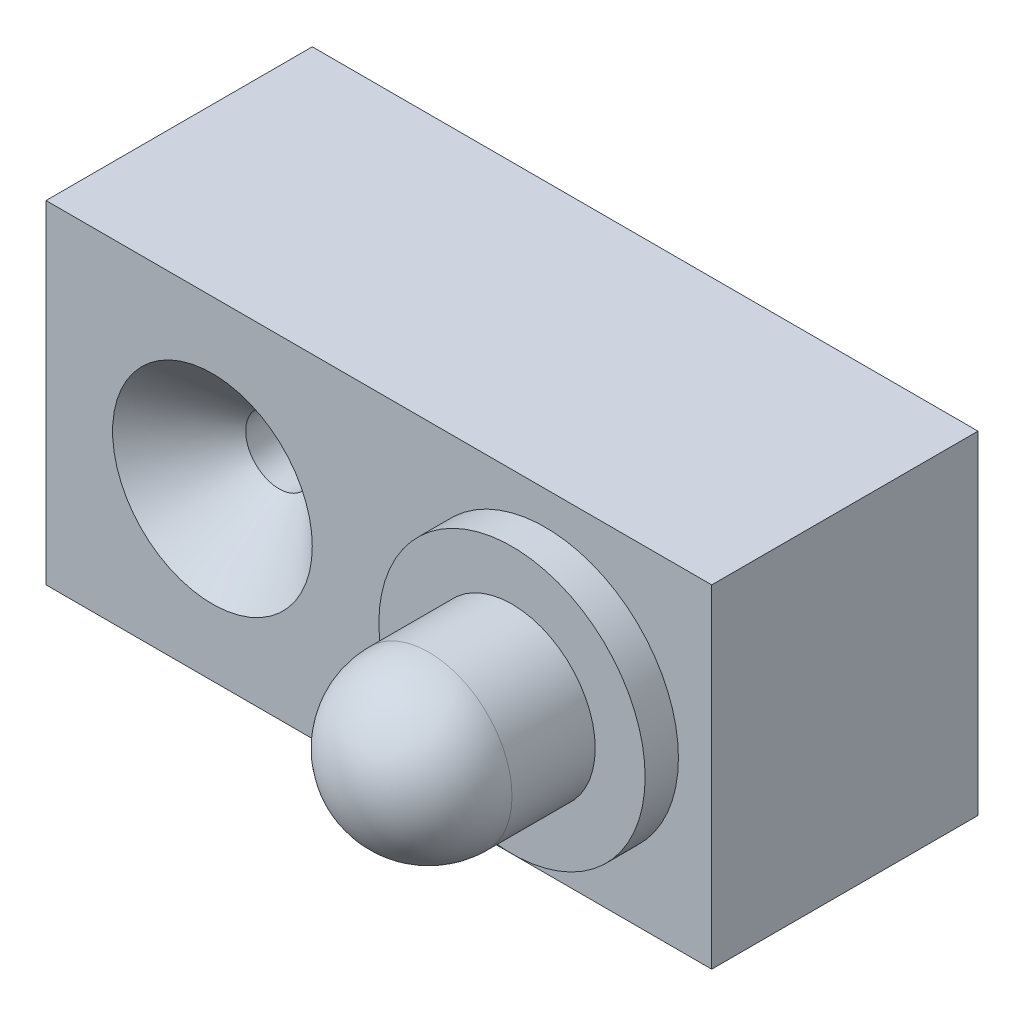
from build123d import *

# Parameters (mm, degrees)
SKETCH_1_W          = 20
SKETCH_1_H          = 10
EXTRUDE_1_DEPTH     = 8
SKETCH_2_R          = 1
CUT_EXTRUDE_1_DEPTH = 8
CHAMFER_1_SIZE      = 2
SKETCH_3_R          = 4
EXTRUDE_2_DEPTH     = 1
SKETCH_4_R          = 2.5
EXTRUDE_3_DEPTH     = 5
FILLET_1_R          = 2.5


with BuildPart() as part:
    # 草图1 → 凸台-拉伸1 (new body)
    with BuildSketch(Plane.XY):
        with Locations((10, 5)):
            Rectangle(SKETCH_1_W, SKETCH_1_H)
    extrude(amount=EXTRUDE_1_DEPTH)

    # 草图2 → 切除-拉伸1 (cut)
    with BuildSketch(Plane.XY.offset(8)):
        with Locations((5, 5)):
            Circle(SKETCH_2_R)
    extrude(amount=-CUT_EXTRUDE_1_DEPTH, mode=Mode.SUBTRACT)

    # 倒角1
    chamfer_1_edges = [part.edges().sort_by_distance(p)[0] for p in [
        (4, 5, 8),
    ]]
    chamfer(chamfer_1_edges, length=CHAMFER_1_SIZE)

    # 草图3 → 凸台-拉伸2 (add)
    with BuildSketch(Plane.XY.offset(8)):
        with Locations(Location((15, 5, 0), (0, 0, 180))):
            Circle(SKETCH_3_R)
    extrude(amount=EXTRUDE_2_DEPTH)

    # 草图4 → 凸台-拉伸3 (add)
    with BuildSketch(Plane.XY.offset(9)):
        with Locations((15, 5)):
            Circle(SKETCH_4_R)
    extrude(amount=EXTRUDE_3_DEPTH)

    # 圆角1
    fillet_1_edges = [part.edges().sort_by_distance(p)[0] for p in [
        (12.5, 5, 14),
    ]]
    fillet(fillet_1_edges, radius=FILLET_1_R)


solid = part.part
